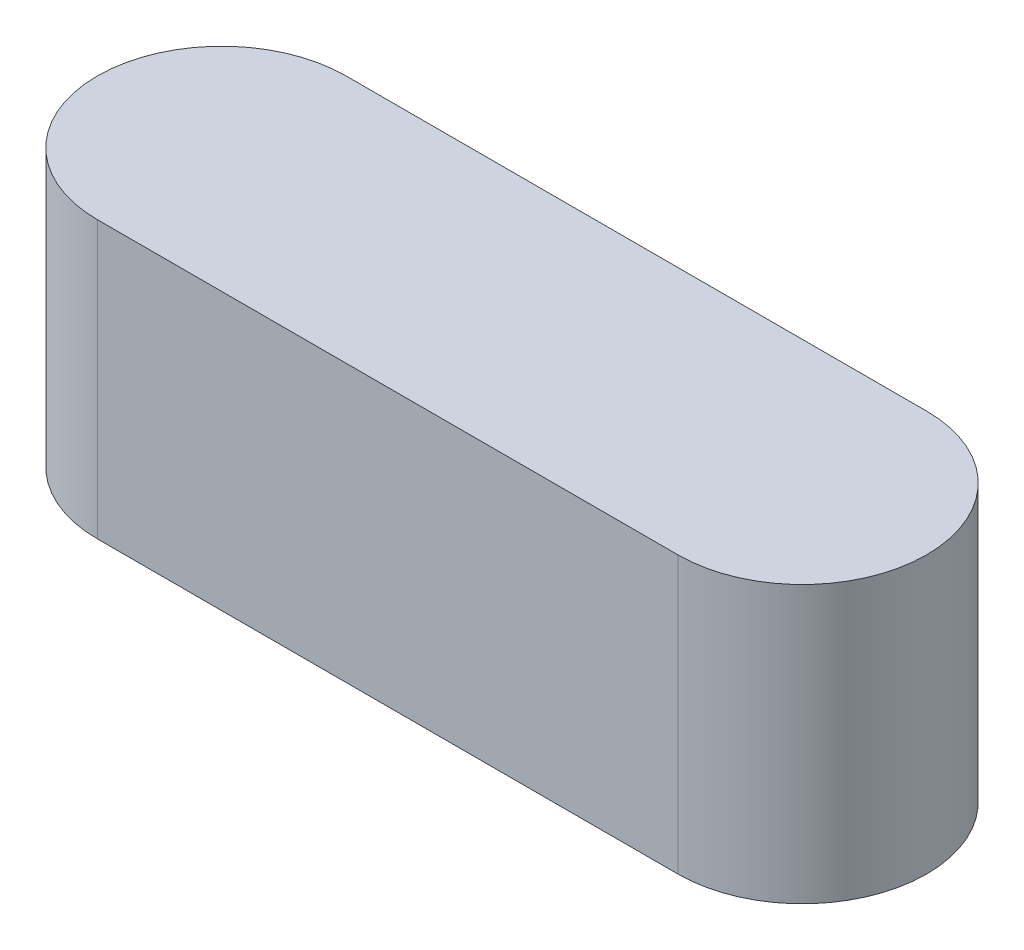
from build123d import *

# Parameters (mm, degrees)
BOSS_EXTRUDE1_DEPTH = 10
SCALE_1_SCALE       = 1.875


with BuildPart() as part:
    # Sketch1 → Boss-Extrude1 (new body)
    with BuildSketch(Plane(origin=(0, 0, 0), x_dir=(1, 0, 0), z_dir=(0, 1, 0))):
        with BuildLine():
            Line((0, 4.5), (21, 4.5))
            ThreePointArc((21, 4.5), (25.5, 0), (21, -4.5))
            Line((21, -4.5), (0, -4.5))
            ThreePointArc((0, -4.5), (-4.5, 0), (0, 4.5))
        make_face()
    extrude(amount=BOSS_EXTRUDE1_DEPTH)


with BuildPart() as part_1:
    # Scale 1: scaled about (10.5, 5, 0)
    add(part.part.scale(SCALE_1_SCALE).moved(Location((-9.1875, -4.375, 0))))


solid = part_1.part
